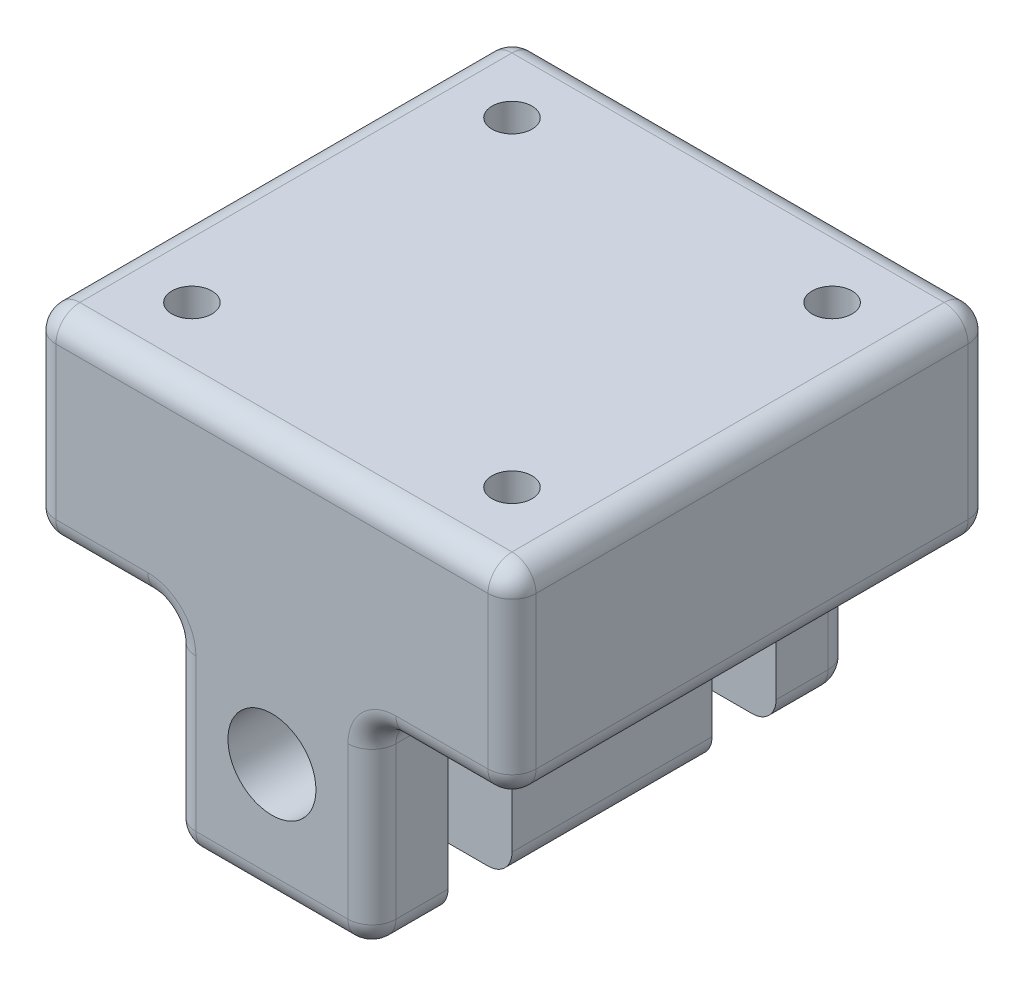
from build123d import *

# Parameters (mm, degrees)
SKETCH1_W           = 17.5
SKETCH1_H           = 25
SKETCH1_W_2         = 12.5
BOSS_EXTRUDE1_DEPTH = 30
FILLET1_R           = 3
SKETCH2_W           = 25
SKETCH2_H           = 8
CUT_EXTRUDE1_DEPTH  = 23
SKETCH3_R           = 2.5
CUT_EXTRUDE2_DEPTH  = 50.244289009


with BuildPart() as part:
    # Sketch1 → Boss-Extrude1 (new, symmetric)
    with BuildSketch(Plane.XY):
        with BuildLine():
            Line((-12.5, 0), (0, 0))
            Line((0, 0), (0, 9.5))
            ThreePointArc((0, 9.5), (-5.5, 15), (0, 20.5))
            Line((0, 20.5), (0, 25))
            Line((0, 25), (-12.5, 25))
            Line((-12.5, 25), (-12.5, 0))
        make_face()
        with BuildLine():
            Line((0, 9.5), (0, 0))
            Line((0, 0), (12.5, 0))
            Line((12.5, 0), (12.5, 25))
            Line((12.5, 25), (0, 25))
            Line((0, 25), (0, 20.5))
            ThreePointArc((0, 20.5), (3.889087297, 18.889087297), (5.5, 15))
            ThreePointArc((5.5, 15), (3.889087297, 11.110912703), (0, 9.5))
        make_face()
        with Locations((21.25, 37.5)):
            Rectangle(SKETCH1_W, SKETCH1_H)
        with Locations((6.25, 37.5)):
            Rectangle(SKETCH1_W_2, SKETCH1_H)
        with Locations((-6.25, 37.5)):
            Rectangle(SKETCH1_W_2, SKETCH1_H)
        with Locations((-21.25, 37.5)):
            Rectangle(SKETCH1_W, SKETCH1_H)
    extrude(amount=BOSS_EXTRUDE1_DEPTH, both=True)

    # Fillet1
    fillet1_edges = [part.edges().sort_by_distance(p)[0] for p in [
        (0, 0, -30),
        (-12.5, 12.5, -30),
        (-21.25, 25, -30),
        (-30, 37.5, -30),
        (30, 37.5, 30),
        (0, 50, -30),
        (30, 37.5, -30),
        (21.25, 25, -30),
        (12.5, 12.5, -30),
        (0, 50, 30),
        (12.5, 0, 0),
        (-12.5, 0, 0),
        (-12.5, 25, 0),
        (-30, 25, 0),
        (-30, 50, 0),
        (30, 50, 0),
        (30, 25, 0),
        (12.5, 25, 0),
        (-30, 37.5, 30),
        (-21.25, 25, 30),
        (-12.5, 12.5, 30),
        (0, 0, 30),
        (12.5, 12.5, 30),
        (21.25, 25, 30),
    ]]
    fillet(fillet1_edges, radius=FILLET1_R)

    # Sketch2 → Cut-Extrude1 (cut)
    with BuildSketch(Plane.XZ):
        with Locations((0, 16.5)):
            Rectangle(SKETCH2_W, SKETCH2_H)
        with Locations((0, -16.5)):
            Rectangle(SKETCH2_W, SKETCH2_H)
    extrude(amount=-CUT_EXTRUDE1_DEPTH, mode=Mode.SUBTRACT)

    # Sketch3 → Cut-Extrude2 (cut, through all)
    with BuildSketch(Plane.XZ.offset(-25)):
        with Locations(Location((20, 20, 0), (0, 0, 270))):
            Circle(SKETCH3_R)
        with Locations(Location((20, -20, 0), (0, 0, 270))):
            Circle(SKETCH3_R)
        with Locations(Location((-20, -20, 0), (0, 0, 270))):
            Circle(SKETCH3_R)
        with Locations(Location((-20, 20, 0), (0, 0, 270))):
            Circle(SKETCH3_R)
    extrude(amount=-CUT_EXTRUDE2_DEPTH, mode=Mode.SUBTRACT)


solid = part.part
